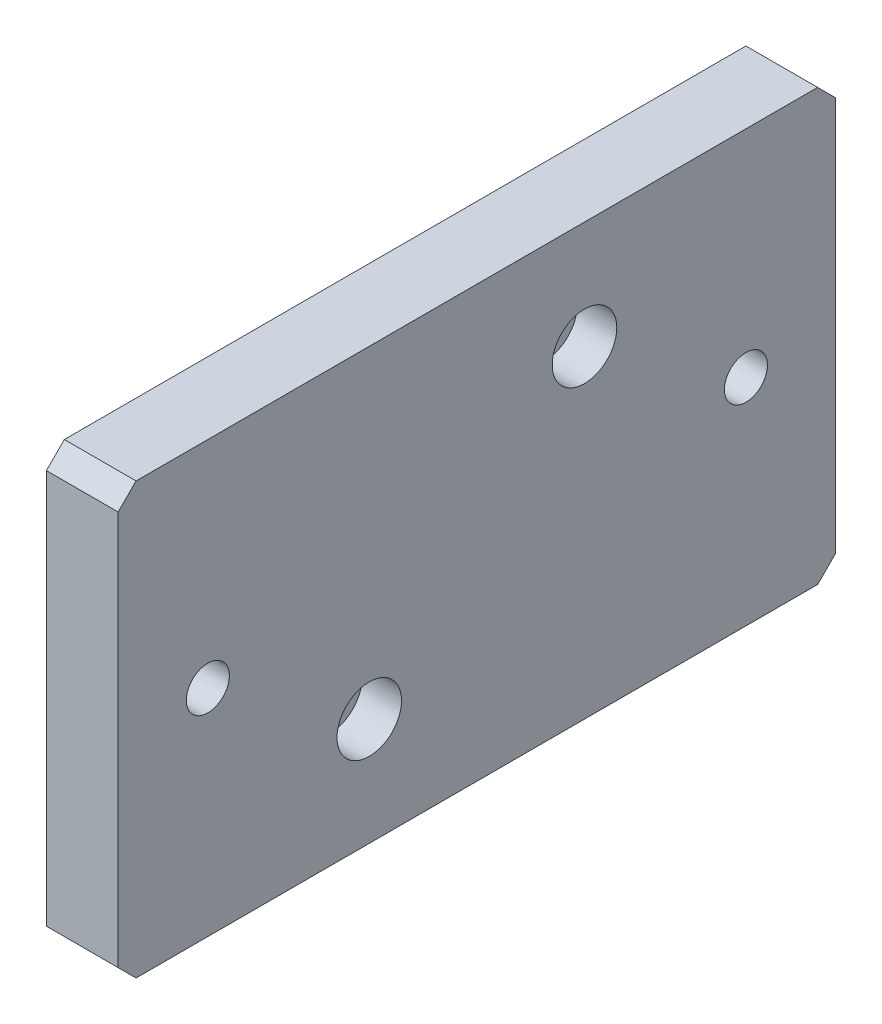
SolidWorks part; units mm, degrees
ref_plane "前视基准面" through (0, 0, 0) normal (0, 0, 1) x (1, 0, 0)
ref_plane "上视基准面" through (0, 0, 0) normal (0, 1, 0) x (1, 0, 0)
ref_plane "右视基准面" through (0, 0, 0) normal (1, 0, 0) x (0, 0, -1)
sketch "草图1" plane through (0, 0, 0) normal (1, 0, 0) x (0, 0, -1)
  line L1 (-100, 60) -> (100, 60)
  line L2 (-100, 60) -> (-100, -60)
  line L3 (-100, -60) -> (100, -60)
  line L4 (100, 60) -> (100, -60)
  line L5 (-100, 60) -> (100, -60) construction
  line L6 (-100, -60) -> (100, 60) construction
  point P0 (0, 0)
  dimension "D1" = 200
  dimension "D2" = 120
extrude "凸台-拉伸1" add sketch "草图1" along normal blind 20
hole_wizard "打孔尺寸(%根据)内六角圆柱头螺钉的类型1" positions "草图2" profile "草图3" counterbore size "M10" standard "GB" end condition through all
sketch "草图2" plane through (20, 0, 0) normal (1, 0, 0) x (0, 0, -1)
  point P0 (30, 30)
  point P2 (-30, -30)
  dimension "D1" = 30
  dimension "D2" = 30
  dimension "D3" = 30
  dimension "D4" = 30
sketch "草图3" plane through (20, 30, -30) normal (0, 1, 0) x (0, 0, -1)
  line L0 (0, 0) -> (0, 20)
  line L1 (0, 20) -> (5.5, 20)
  line L3 (5.5, 20) -> (5.5, 11)
  line L4 (5.5, 11) -> (9, 11)
  line L5 (9, 11) -> (9, 0)
  line L7 (9, 0) -> (0, 0)
  line L11 (0, -6.35) -> (0, 107.95) construction
  dimension "通孔孔直径" = 11
  dimension "通孔孔深度" = 20
  dimension "柱形沉头孔直径" = 18
  dimension "柱形沉头孔深度" = 11
hole_wizard "M14 螺纹孔1" positions "草图4" profile "草图5" tap size "M14" standard "GB" end condition through all
sketch "草图4" plane through (20, 0, 0) normal (1, 0, 0) x (0, 0, -1)
  line L0 (-100, 0) -> (127.5725, 0) construction
  line L1 (-100, 60) -> (-100, -60) construction
  line L3 (0, 0) -> (0, 63.8775) construction
  point P0 (-75, 0)
  point P2 (75, 0)
  dimension "D1" = 150
sketch "草图5" plane through (20, 0, 75) normal (0, 1, 0) x (0, 0, -1)
  line L0 (0, 0) -> (0, 20)
  line L1 (0, 20) -> (6, 20)
  line L2 (6, 20) -> (6, 0)
  line L5 (6, 0) -> (0, 0)
  line L11 (0, -6.35) -> (0, 107.95) construction
  dimension "通孔螺纹孔钻头直径" = 12
  dimension "通孔螺纹孔钻头深度" = 20
cosmetic thread "孔螺蚊线1"
cosmetic thread "孔螺蚊线2"
chamfer "倒角1" distance 5 angle 45 4 edges at (10, 60, 100) (10, 60, -100) (10, -60, -100) (10, -60, 100)
